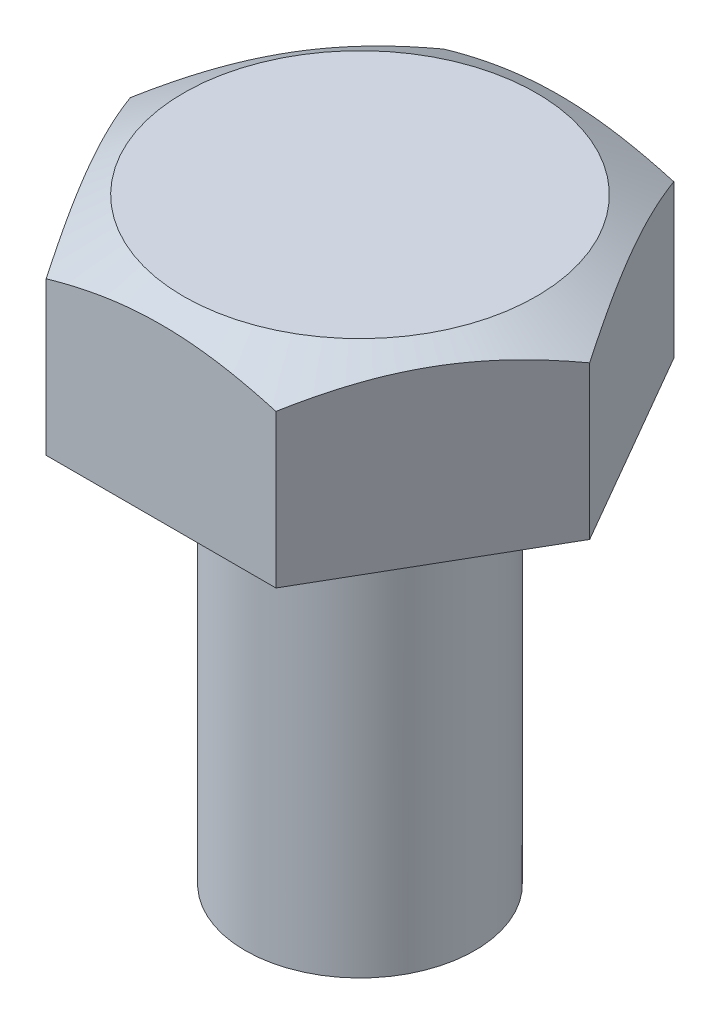
SolidWorks part; units mm, degrees
ref_plane "Front Plane" through (0, 0, 0) normal (0, 0, 1) x (1, 0, 0)
ref_plane "Top Plane" through (0, 0, 0) normal (0, 1, 0) x (1, 0, 0)
ref_plane "Right Plane" through (0, 0, 0) normal (1, 0, 0) x (0, 0, -1)
sketch "Sketch1" plane through (0, 0, 0) normal (0, 1, 0) x (1, 0, 0)
  line L1 (5, 0) -> (2.5, 4.3301)
  line L2 (2.5, 4.3301) -> (-2.5, 4.3301)
  line L3 (-2.5, 4.3301) -> (-5, 0)
  line L4 (-5, 0) -> (-2.5, -4.3301)
  line L5 (-2.5, -4.3301) -> (2.5, -4.3301)
  line L6 (2.5, -4.3301) -> (5, 0)
  circle A0 centre (0, 0) radius 4.3301 construction
  dimension "D1" = 10
extrude "Boss-Extrude1" add sketch "Sketch1" along normal blind 4
sketch "Sketch2" plane through (0, 4, 0) normal (0, 1, 0) x (1, 0, 0)
  circle A0 centre (0, 0) radius 3.8386
extrude "Cut-Extrude1" cut sketch "Sketch2" against normal through all draft 60 flip side to cut
sketch "Sketch3" plane through (0, 0, 0) normal (0, -1, 0) x (1, 0, 0)
  circle A0 centre (0, 0) radius 2.5
  dimension "D1" = 5
extrude "Boss-Extrude2" add sketch "Sketch3" along normal blind 9
